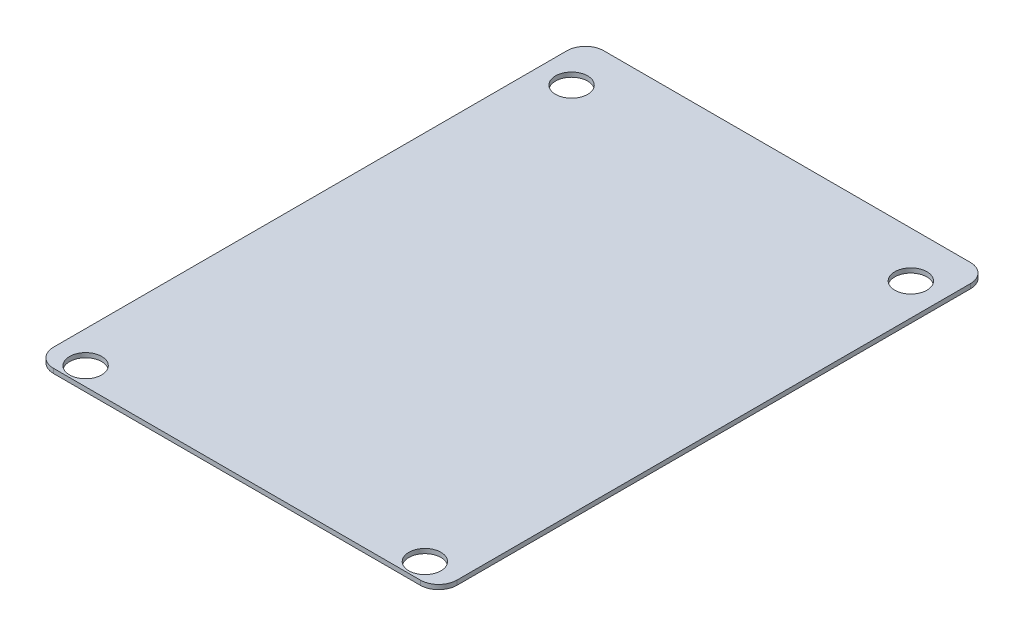
from build123d import *

# Parameters (mm, degrees)
SKETCH1_W                      = 139.7
SKETCH1_H                      = 190.5
BOSS_EXTRUDE1_DEPTH            = 1.5748
FILLET1_R                      = 6.35
F_7_16_0_4375_DIAMETER_HOLE1_D = 11.1125
LPATTERN1_COUNT                = 2
LPATTERN1_PITCH                = 168.275
LPATTERN1_COUNT_DIR2           = 2
LPATTERN1_PITCH_DIR2           = 117.475


with BuildPart() as part:
    # Sketch1 → Boss-Extrude1 (new body)
    with BuildSketch(Plane(origin=(0, 0, 0), x_dir=(1, 0, 0), z_dir=(0, 1, 0))):
        with Locations((0, 4.7625)):
            Rectangle(SKETCH1_W, SKETCH1_H)
    extrude(amount=BOSS_EXTRUDE1_DEPTH)

    # Fillet1
    fillet1_edges = [part.edges().sort_by_distance(p)[0] for p in [
        (-69.85, 0.7874, -100.0125),
        (69.85, 0.7874, -100.0125),
        (69.85, 0.7874, 90.4875),
        (-69.85, 0.7874, 90.4875),
    ]]
    fillet(fillet1_edges, radius=FILLET1_R)

    # 7/16 (0.4375) Diameter Hole1 (through all)
    with Locations(Plane(origin=(0, 1.5748, 0), x_dir=(1, 0, 0), z_dir=(0, 1, 0))):
        with Locations((-58.738, 84.1375)):
            f_7_16_0_4375_diameter_hole1 = Hole(F_7_16_0_4375_DIAMETER_HOLE1_D / 2)

    # LPattern1: 7_16 _0.4375_ Diameter Hole1 2 × 2
    with Locations(*[(j * LPATTERN1_PITCH_DIR2, 0, i * LPATTERN1_PITCH) for i in range(LPATTERN1_COUNT) for j in range(LPATTERN1_COUNT_DIR2) if (i, j) != (0, 0)]):
        add(f_7_16_0_4375_diameter_hole1, mode=Mode.SUBTRACT)


solid = part.part
